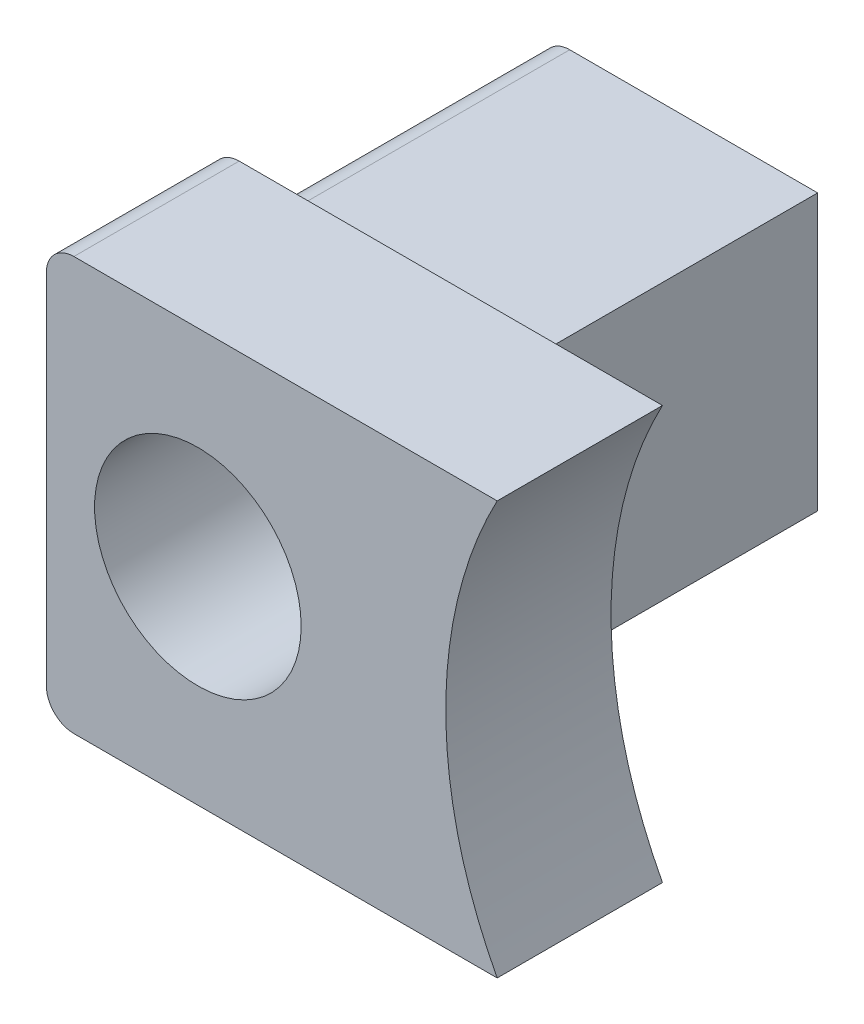
from build123d import *

# Parameters (mm, degrees)
SKETCH1_W                                           = 16.5
SKETCH1_H                                           = 15
BOSS_EXTRUDE1_DEPTH                                 = 18
FILLET1_R                                           = 1
CBORE_FOR_M4_HEX_SOCKET_HEAD_CAP_SCREW1_D           = 4.5
CBORE_FOR_M4_HEX_SOCKET_HEAD_CAP_SCREW1_CBORE_D     = 7.5
CBORE_FOR_M4_HEX_SOCKET_HEAD_CAP_SCREW1_CBORE_DEPTH = 8
SKETCH7_R                                           = 16
CUT_EXTRUDE2_DEPTH                                  = 22.17339132
SKETCH8_W                                           = 6.5
SKETCH8_H                                           = 12
CUT_EXTRUDE3_DEPTH                                  = 25.840742743
SKETCH9_W                                           = 10
SKETCH9_H                                           = 12
CUT_EXTRUDE4_DEPTH                                  = 2.5
FILLET2_R                                           = 1


with BuildPart() as part:
    # Sketch1 → Boss-Extrude1 (new body)
    with BuildSketch(Plane.XY):
        Rectangle(SKETCH1_W, SKETCH1_H)
    extrude(amount=BOSS_EXTRUDE1_DEPTH)

    # Fillet1
    fillet1_edges = [part.edges().sort_by_distance(p)[0] for p in [
        (-8.25, -7.5, 9),
        (-8.25, 7.5, 9),
    ]]
    fillet(fillet1_edges, radius=FILLET1_R)

    # CBORE for M4 Hex Socket Head Cap Screw1 (through all)
    with Locations(Plane.XY.offset(18)):
        with Locations((-2.75, 0)):
            CounterBoreHole(CBORE_FOR_M4_HEX_SOCKET_HEAD_CAP_SCREW1_D / 2, CBORE_FOR_M4_HEX_SOCKET_HEAD_CAP_SCREW1_CBORE_D / 2, CBORE_FOR_M4_HEX_SOCKET_HEAD_CAP_SCREW1_CBORE_DEPTH)

    # Sketch7 → Cut-Extrude2 (cut, through all)
    with BuildSketch(Plane.XY.offset(18)):
        with Locations((22.25, 0)):
            Circle(SKETCH7_R)
    extrude(amount=-CUT_EXTRUDE2_DEPTH, mode=Mode.SUBTRACT)

    # Sketch8 → Cut-Extrude3 (cut, through all)
    with BuildSketch(Plane(origin=(0, 7.5, 0), x_dir=(1, 0, 0), z_dir=(0, 1, 0))):
        with Locations((5, -6)):
            Rectangle(SKETCH8_W, SKETCH8_H)
    extrude(amount=-CUT_EXTRUDE3_DEPTH, mode=Mode.SUBTRACT)

    # Sketch9 → Cut-Extrude4 (cut)
    with BuildSketch(Plane(origin=(0, -7.5, 0), x_dir=(-1, 0, 0), z_dir=(0, -1, 0))):
        with Locations((3.25, -6)):
            Rectangle(SKETCH9_W, SKETCH9_H)
    cut_extrude4 = extrude(amount=-CUT_EXTRUDE4_DEPTH, mode=Mode.SUBTRACT)

    # Mirror1: Cut-Extrude4 across plane
    add(cut_extrude4.mirror(Plane.ZX), mode=Mode.SUBTRACT)

    # Fillet2
    fillet2_edges = [part.edges().sort_by_distance(p)[0] for p in [
        (-8.25, 5, 6),
        (-8.25, -5, 6),
    ]]
    fillet(fillet2_edges, radius=FILLET2_R)


solid = part.part
